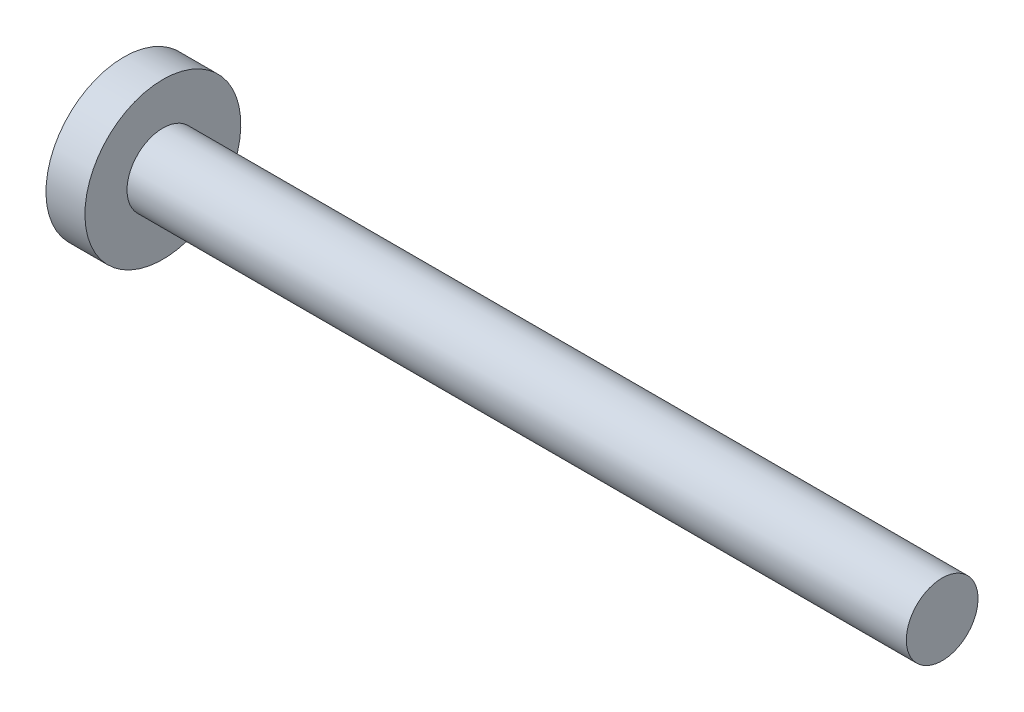
from build123d import *

# Parameters (mm, degrees)
CUT_EXTRUDE1_DEPTH = 2.54
FILLET2_R          = 0.8128


with BuildPart() as part:
    # Sketch1 → Revolve1 (revolve)
    with BuildSketch(Plane.XY):
        Polygon((0, 5.842), (0, 12.7), (-6.35, 12.7), (-6.35, 0), (0, 0), (127, 0), (127, 5.842), align=None)
    revolve(axis=Axis((127, 0, 0), (-1, 0, 0)))

    # Sketch2 → Cut-Extrude1 (cut)
    with BuildSketch(Plane.ZY.offset(6.35)):
        Polygon((-2.54, 6.35), (-2.54, 2.54), (-6.35, 2.54), (-6.35, -2.54), (-2.54, -2.54), (-2.54, -6.122575092), (2.54, -6.122575092), (2.54, -2.54), (6.35, -2.54), (6.35, 2.54), (2.54, 2.54), (2.54, 6.35), align=None)
    extrude(amount=-CUT_EXTRUDE1_DEPTH, mode=Mode.SUBTRACT)

    # Fillet2
    fillet2_edges = [part.edges().sort_by_distance(p)[0] for p in [
        (-6.35, 6.35, 0),
        (-6.35, 4.445, -2.54),
        (-6.35, 2.54, -4.445),
        (-6.35, 0, -6.35),
        (-6.35, -2.54, -4.445),
        (-6.35, -4.331287546, -2.54),
        (-6.35, -6.122575092, 0),
        (-6.35, -4.331287546, 2.54),
        (-6.35, -2.54, 4.445),
        (-6.35, 0, 6.35),
        (-6.35, 2.54, 4.445),
        (-6.35, 4.445, 2.54),
    ]]
    fillet(fillet2_edges, radius=FILLET2_R)


solid = part.part
